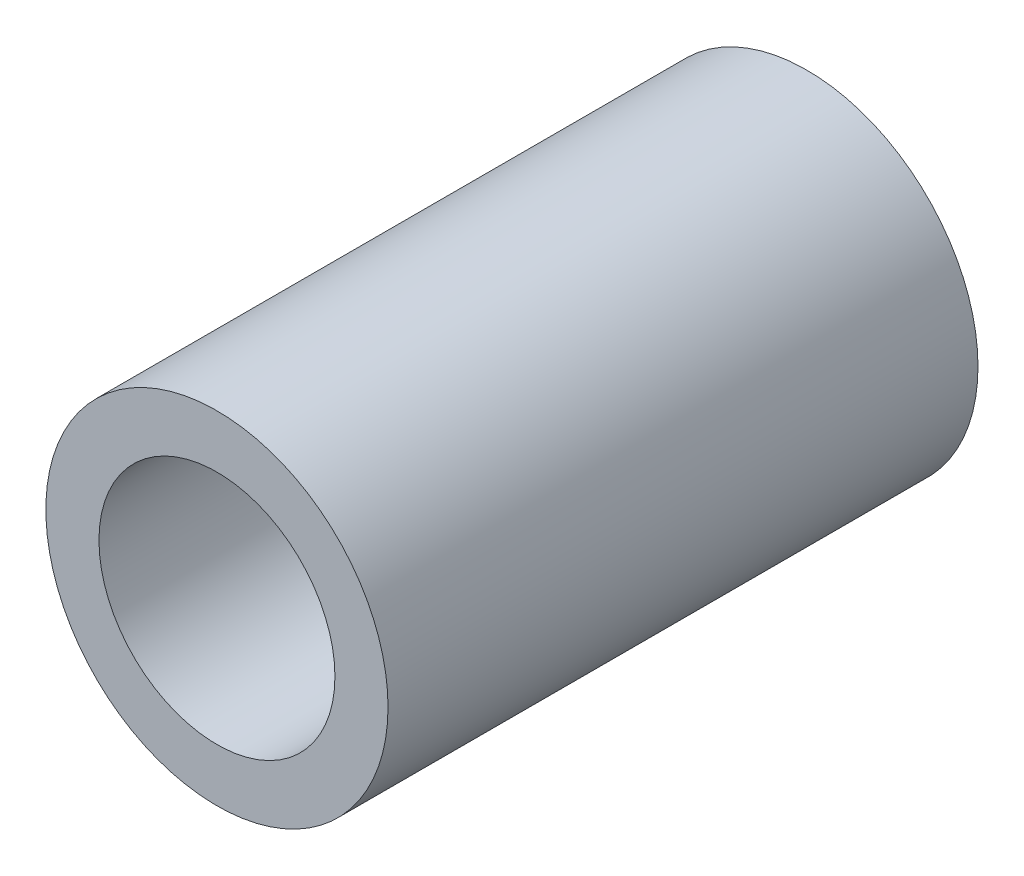
SolidWorks part; units mm, degrees
ref_plane "前视基准面" through (0, 0, 0) normal (0, 0, 1) x (1, 0, 0)
ref_plane "上视基准面" through (0, 0, 0) normal (0, 1, 0) x (1, 0, 0)
ref_plane "右视基准面" through (0, 0, 0) normal (1, 0, 0) x (0, 0, -1)
sketch "草图1" plane through (0, 0, 0) normal (0, 0, 1) x (1, 0, 0)
  circle A0 centre (0, 0) radius 14.5
  circle A1 centre (0, 0) radius 10
  dimension "D1" = 29
  dimension "D2" = 20
extrude "凸台-拉伸1" add sketch "草图1" along normal blind 50
cosmetic thread "装饰螺纹线1" parameters "D1"=20, "D2"=21
